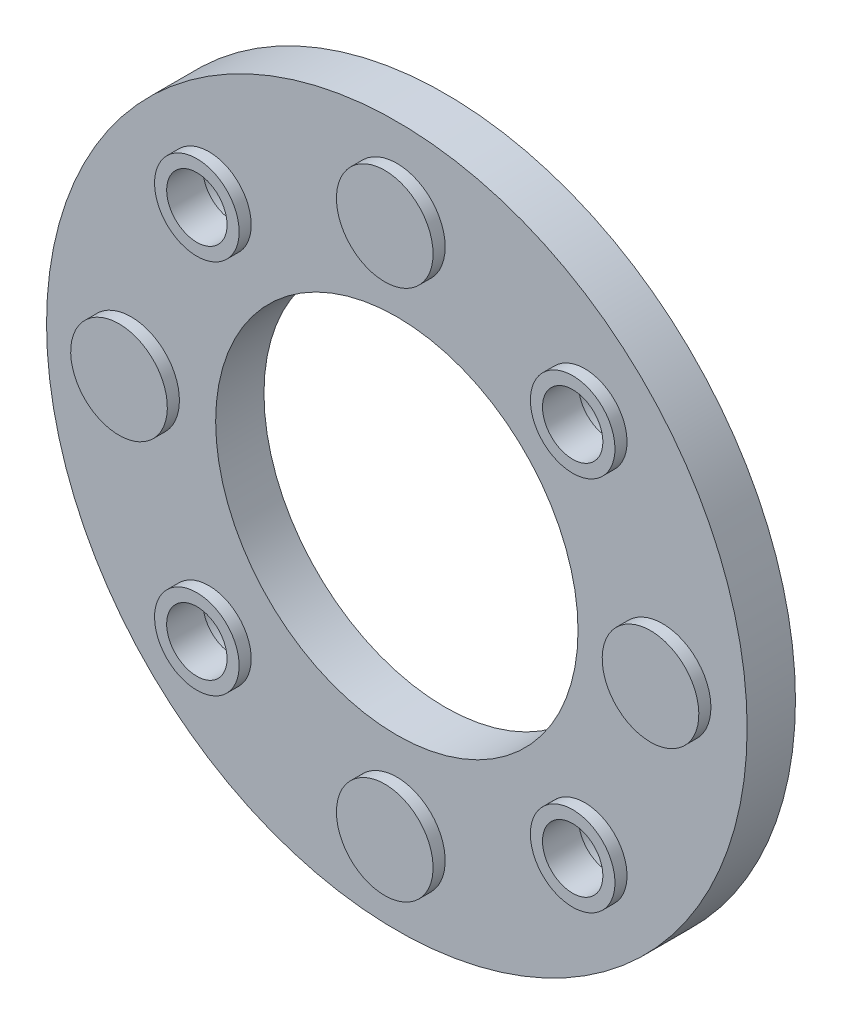
from build123d import *

# Parameters (mm, degrees)
SKETCH1_R           = 29
BOSS_EXTRUDE1_DEPTH = 4
SKETCH2_R           = 15
CUT_EXTRUDE1_DEPTH  = 24
SKETCH3_R           = 4
BOSS_EXTRUDE2_DEPTH = 1
SKETCH5_R           = 2.5
CUT_EXTRUDE2_DEPTH  = 4.5
CIRPATTERN1_COUNT   = 4
SKETCH6_R           = 3.5
BOSS_EXTRUDE3_DEPTH = 1
SKETCH7_R           = 3.5
CUT_EXTRUDE3_DEPTH  = 2
SKETCH8_R           = 2.5
CUT_EXTRUDE4_DEPTH  = 10
CIRPATTERN2_COUNT   = 4


with BuildPart() as part:
    # Sketch1 → Boss-Extrude1 (new body)
    with BuildSketch(Plane.XY):
        Circle(SKETCH1_R)
    extrude(amount=BOSS_EXTRUDE1_DEPTH)

    # Sketch2 → Cut-Extrude1 (cut)
    with BuildSketch(Plane.XY.offset(4)):
        Circle(SKETCH2_R)
    extrude(amount=-CUT_EXTRUDE1_DEPTH, mode=Mode.SUBTRACT)

    # Sketch3 → Boss-Extrude2 (add)
    with BuildSketch(Plane.XY.offset(4)):
        with Locations((0, 22)):
            Circle(SKETCH3_R)
    boss_extrude2 = extrude(amount=BOSS_EXTRUDE2_DEPTH)

    # Sketch5 → Cut-Extrude2 (cut)
    with BuildSketch(Plane(origin=(0, 0, 0), x_dir=(-1, 0, 0), z_dir=(0, 0, -1))):
        with Locations((0, 22)):
            Circle(SKETCH5_R)
    cut_extrude2 = extrude(amount=-CUT_EXTRUDE2_DEPTH, mode=Mode.SUBTRACT)

    # CirPattern1: Boss-Extrude2, Cut-Extrude2 ×4 about axis
    cirpattern1_axis = Axis((0, 0, 0), (0, 0, 1))
    add([boss_extrude2.rotate(cirpattern1_axis, i * 360 / CIRPATTERN1_COUNT) for i in range(1, CIRPATTERN1_COUNT)])
    add([cut_extrude2.rotate(cirpattern1_axis, i * 360 / CIRPATTERN1_COUNT) for i in range(1, CIRPATTERN1_COUNT)], mode=Mode.SUBTRACT)

    # Sketch6 → Boss-Extrude3 (add)
    with BuildSketch(Plane.XY.offset(4)):
        with Locations((-15.556349186, 15.556349186)):
            Circle(SKETCH6_R)
    boss_extrude3 = extrude(amount=BOSS_EXTRUDE3_DEPTH)

    # Sketch7 → Cut-Extrude3 (cut)
    with BuildSketch(Plane(origin=(0, 0, 0), x_dir=(-1, 0, 0), z_dir=(0, 0, -1))):
        with Locations(Location((15.556349186, 15.556349186, 0), (0, 0, 180))):
            Circle(SKETCH7_R)
    cut_extrude3 = extrude(amount=-CUT_EXTRUDE3_DEPTH, mode=Mode.SUBTRACT)

    # Sketch8 → Cut-Extrude4 (cut)
    with BuildSketch(Plane(origin=(0, 0, 2), x_dir=(-1, 0, 0), z_dir=(0, 0, -1))):
        with Locations((15.556349186, 15.556349186)):
            Circle(SKETCH8_R)
    cut_extrude4 = extrude(amount=-CUT_EXTRUDE4_DEPTH, mode=Mode.SUBTRACT)

    # CirPattern2: Boss-Extrude3, Cut-Extrude3, Cut-Extrude4 ×4 about axis
    cirpattern2_axis = Axis((0, 0, 0), (0, 0, 1))
    add([boss_extrude3.rotate(cirpattern2_axis, i * 360 / CIRPATTERN2_COUNT) for i in range(1, CIRPATTERN2_COUNT)])
    add([cut_extrude3.rotate(cirpattern2_axis, i * 360 / CIRPATTERN2_COUNT) for i in range(1, CIRPATTERN2_COUNT)], mode=Mode.SUBTRACT)
    add([cut_extrude4.rotate(cirpattern2_axis, i * 360 / CIRPATTERN2_COUNT) for i in range(1, CIRPATTERN2_COUNT)], mode=Mode.SUBTRACT)


solid = part.part
